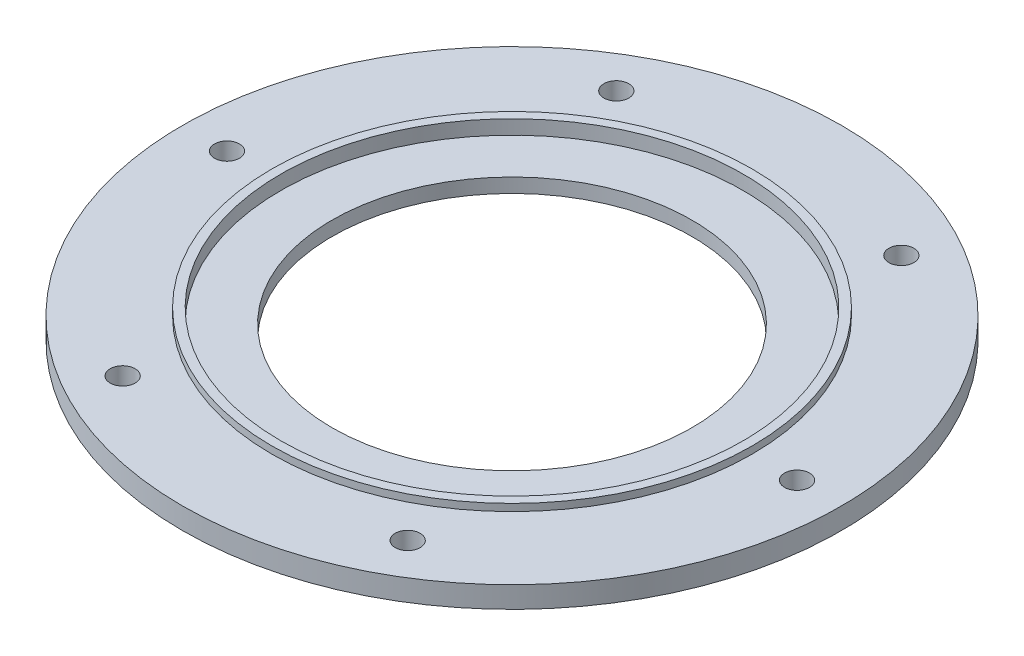
SolidWorks part; units mm, degrees
material "Gray Cast Iron"
ref_plane "Front Plane" through (0, 0, 0) normal (0, 0, 1) x (1, 0, 0)
ref_plane "Top Plane" through (0, 0, 0) normal (0, 1, 0) x (1, 0, 0)
ref_plane "Right Plane" through (0, 0, 0) normal (1, 0, 0) x (0, 0, -1)
sketch "Sketch1" plane through (0, 0, 0) normal (0, 1, 0) x (1, 0, 0)
  circle A0 centre (0, 0) radius 185
  circle A1 centre (0, 0) radius 101
  dimension "D1" = 370
  dimension "D2" = 202
extrude "Boss-Extrude1" add sketch "Sketch1" along normal blind 12
sketch "Sketch2" plane through (0, 12, 0) normal (0, 1, 0) x (1, 0, 0)
  circle A0 centre (0, 0) radius 129.75
  dimension "D1" = 259.5
extrude "Cut-Extrude1" cut sketch "Sketch2" against normal blind 4
sketch "Sketch3" plane through (0, 12, 0) normal (0, 1, 0) x (1, 0, 0)
  circle A0 centre (0, 0) radius 129.75 construction
  circle A1 centre (0, 0) radius 129.75
  circle A2 centre (0, 0) radius 134.75
  dimension "D1" = 269.5
extrude "Boss-Extrude2" add sketch "Sketch3" along normal blind 4
sketch "Sketch4" plane through (0, 12, 0) normal (0, 1, 0) x (1, 0, 0)
  line L0 (0, 0) -> (160, 0) construction
  circle A0 centre (0, 0) radius 160 construction
  circle A1 centre (160, 0) radius 7
  dimension "D1" = 320
  dimension "D2" = 14
extrude "Cut-Extrude2" cut sketch "Sketch4" against normal through all
pattern_circular "CirPattern1" count 6 over 360 about axis through (0, 0, 0) along (0, 1, 0) of "Cut-Extrude2"
